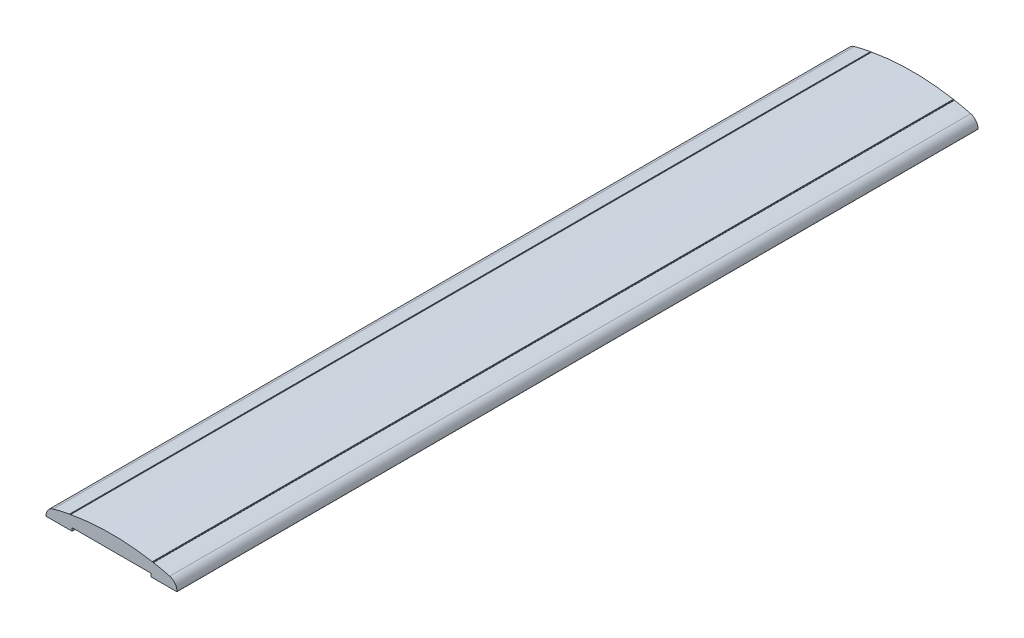
from build123d import *

# Parameters (mm, degrees)
EXTRUDE_1_DEPTH = 575
FILLET_1_R      = 0.3


with BuildPart() as part:
    # 草图1 → 凸台-拉伸1 (new, symmetric)
    with BuildSketch(Plane.XY):
        with BuildLine():
            Line((94, 0), (56.7, 0))
            ThreePointArc((56.7, 0), (56.558578644, 0.058578644), (56.5, 0.2))
            Line((56.5, 0.2), (56.5, 4.5))
            Line((56.5, 4.5), (-56.5, 4.5))
            Line((-56.5, 4.5), (-56.5, 0.2))
            ThreePointArc((-56.5, 0.2), (-56.558578644, 0.058578644), (-56.7, 0))
            Line((-56.7, 0), (-94, 0))
            ThreePointArc((-94, 0), (-91.314648859, 8.987866196), (-83.557929261, 14.262916014))
            ThreePointArc((-83.557929261, 14.262916014), (-72.015896085, 17.05846092), (-60.38087895, 19.437531623))
            ThreePointArc((-60.38087895, 19.437531623), (-60.316820101, 19.428115404), (-60.271957046, 19.381430208))
            ThreePointArc((-60.271957046, 19.381430208), (-59.945537065, 19.213061927), (-59.70074969, 19.486881253))
            ThreePointArc((-59.70074969, 19.486881253), (-59.675512901, 19.546507637), (-59.619038631, 19.578175571))
            ThreePointArc((-59.619038631, 19.578175571), (-59.500070371, 19.599971741), (-59.381094143, 19.621724372))
            ThreePointArc((-59.381094143, 19.621724372), (-59.317064562, 19.612111154), (-59.272345321, 19.565288181))
            ThreePointArc((-59.272345321, 19.565288181), (-58.946444781, 19.395916638), (-58.700816303, 19.668981709))
            ThreePointArc((-58.700816303, 19.668981709), (-58.675396224, 19.728530183), (-58.618824811, 19.760024254))
            ThreePointArc((-58.618824811, 19.760024254), (0, 25), (58.618824811, 19.760024254))
            ThreePointArc((58.618824811, 19.760024254), (58.675396224, 19.728530183), (58.700816303, 19.668981709))
            ThreePointArc((58.700816303, 19.668981709), (58.946444781, 19.395916638), (59.272345321, 19.565288181))
            ThreePointArc((59.272345321, 19.565288181), (59.317064562, 19.612111154), (59.381094143, 19.621724372))
            ThreePointArc((59.381094143, 19.621724372), (59.500070371, 19.599971741), (59.619038631, 19.578175571))
            ThreePointArc((59.619038631, 19.578175571), (59.675512901, 19.546507637), (59.70074969, 19.486881253))
            ThreePointArc((59.70074969, 19.486881253), (59.945537065, 19.213061927), (60.271957046, 19.381430208))
            ThreePointArc((60.271957046, 19.381430208), (60.316820101, 19.428115404), (60.38087895, 19.437531623))
            ThreePointArc((60.38087895, 19.437531623), (72.015896085, 17.05846092), (83.557929261, 14.262916014))
            ThreePointArc((83.557929261, 14.262916014), (91.314648859, 8.987866196), (94, 0))
        make_face()
    extrude(amount=EXTRUDE_1_DEPTH, both=True)

    # 圆角1
    fillet_1_edges = [part.edges().sort_by_distance(p)[0] for p in [
        (94, 0, 0),
        (-94, 0, 0),
    ]]
    fillet(fillet_1_edges, radius=FILLET_1_R)


solid = part.part
